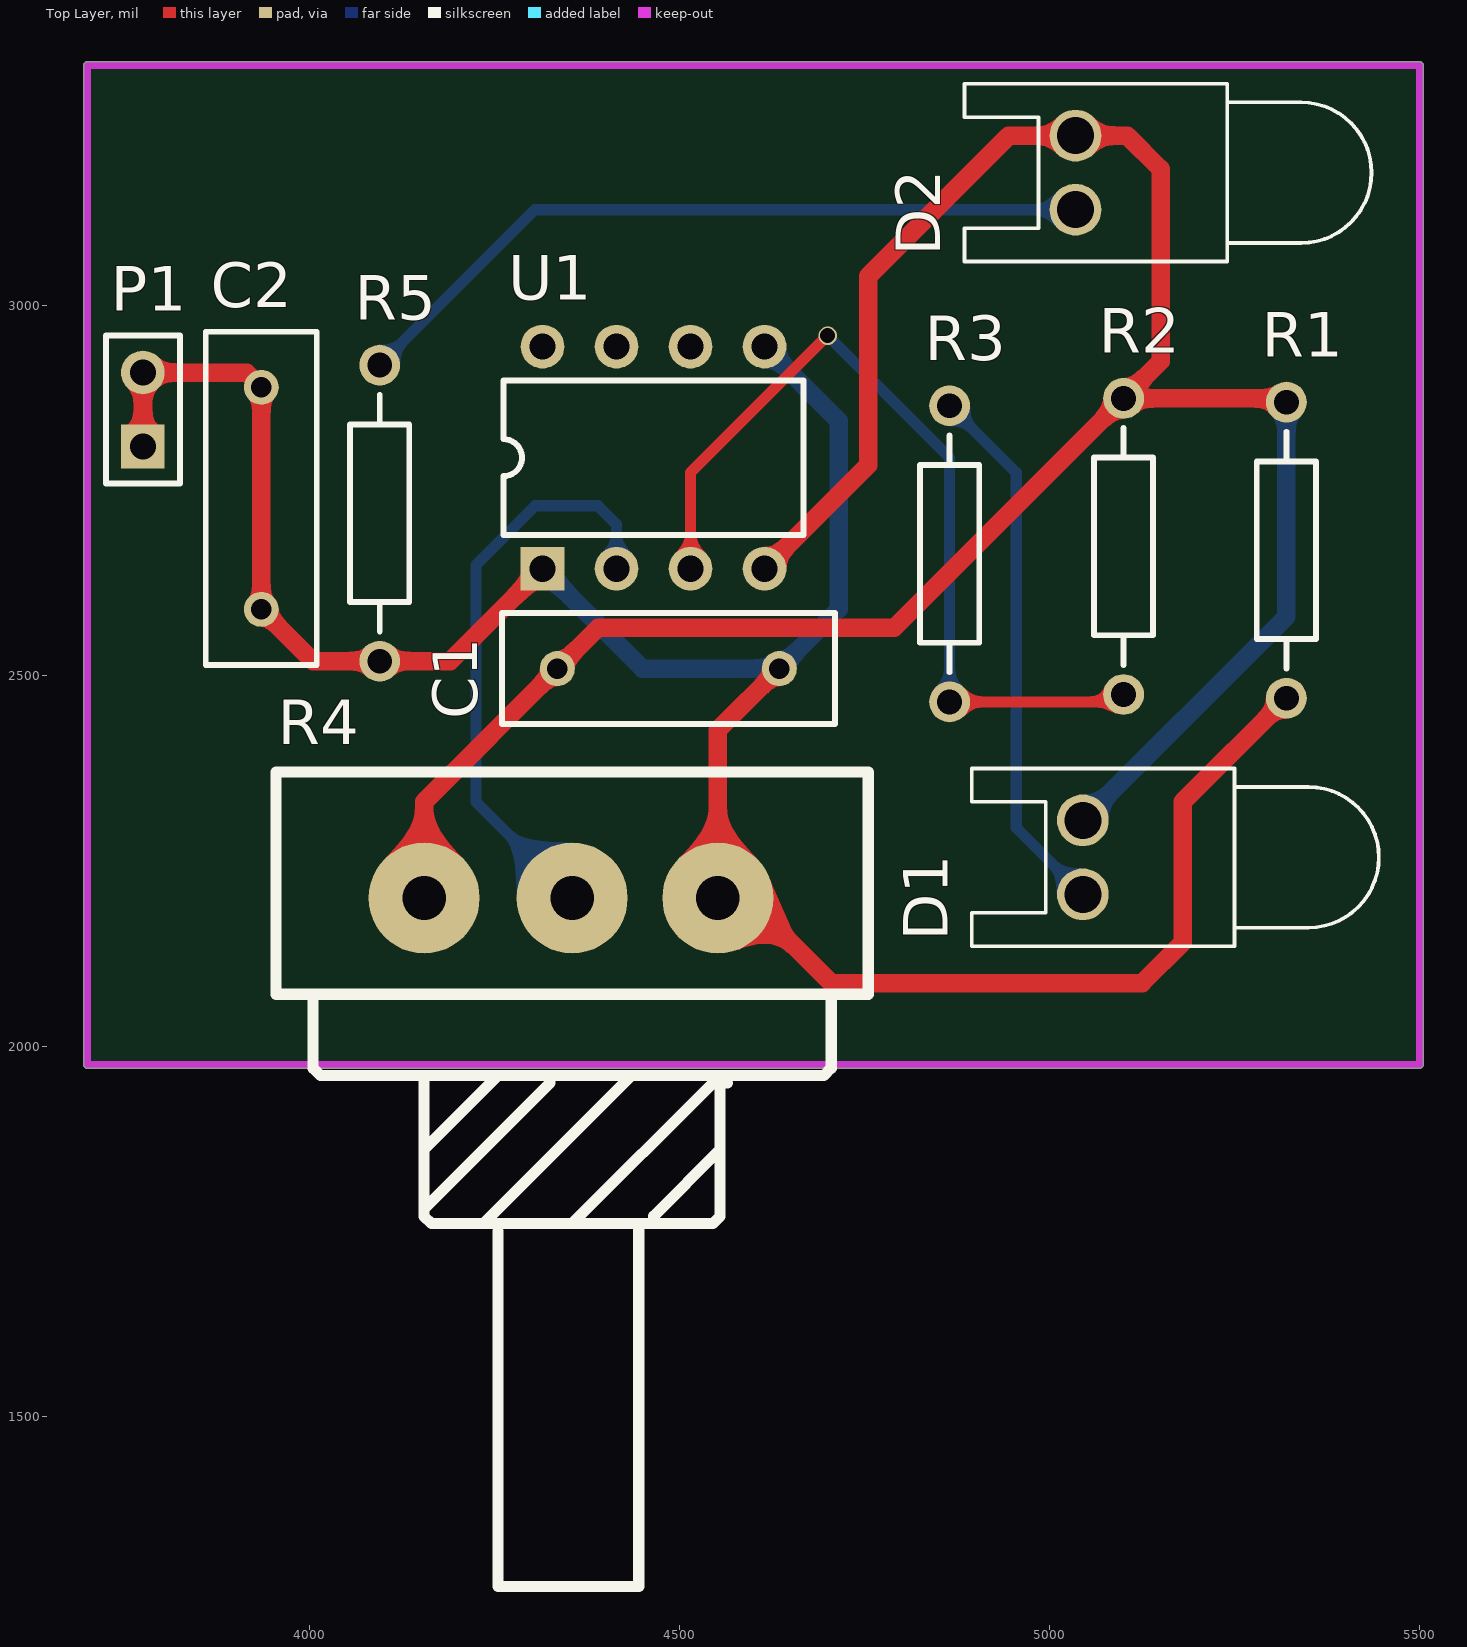
[diagram p0: Top Layer view]
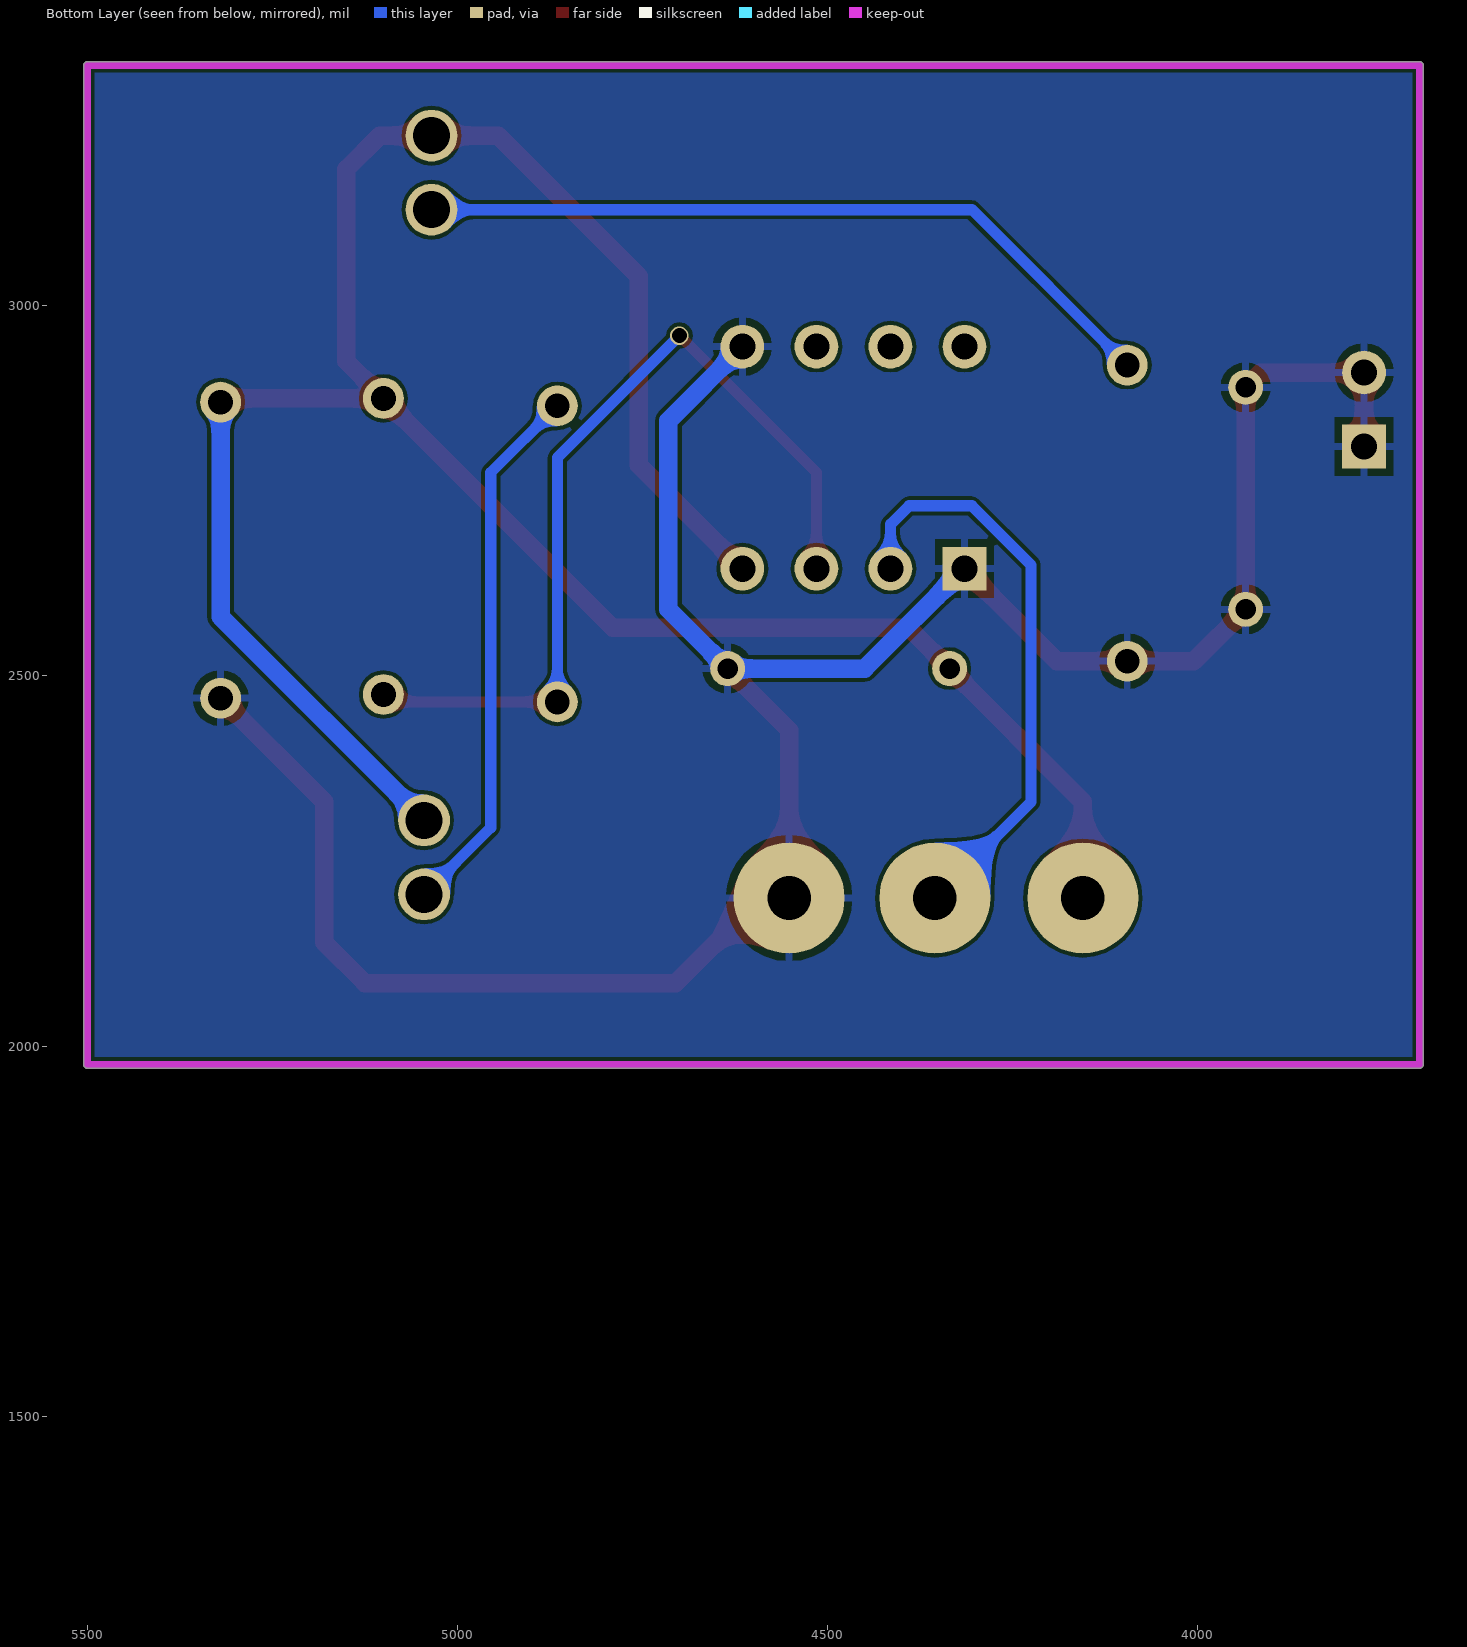
[diagram p1: Bottom Layer view, seen from below]
# Altium PCB MISC82777.PcbDoc
Units mil, origin at the board's own origin, x right, y up, seen from the top; angles counter-clockwise.
Board outline 1810.03 x 1360.03 mil, 2 copper layers (Top Layer, Bottom Layer); 11 components, 6 nets, 29 pads, 1 vias.

## Layer stack, top to bottom (the 12.6 mil dielectric is the usual default, probably not edited)
Top Solder: solder mask 0.4, Solder Resist, Dk 3.5
Top Layer: signal copper 1.4
Dielectric 1: dielectric 12.6, FR-4, Dk 4.8
Bottom Layer: signal copper 1.4
Bottom Solder: solder mask 0.4, Solder Resist, Dk 3.5

## Board outline
3694.99,1975 ccw(c3700,1975) 3700,1969.98 5500,1969.98 ccw(c5500,1975) 5505.02,1975 5505.02,3325 ccw(c5500,3325) 5500,3330.01 3700,3330.01 ccw(c3700,3325) 3694.99,3325

## Design rules (kind name [scope] priority, off if disabled: settings)
Clearance [All] p1: gap=5 ignorepadtopadclearanceinfootprint=FALSE except(0: Arc-Hole Track-Hole SMDPad-Hole THPad-Hole Via-Hole Fill-Hole Poly-Hole Region-Hole Text-Hole)
PolygonConnect [All] p1: connectstyle=Relief reliefconductorwidth=10 reliefentries=4 polygonreliefangle="90 Angle" airgapwidth=10
RoutingVias [All] p1: holewidth=28 width=50 viastyle="Through Hole" minholewidth=28 minwidth=50 maxholewidth=28 maxwidth=50
SolderMaskExpansion [All] p1: expansion=4
Width [All] p1: maxlimit=10000 minlimit=10 preferedwidth=10 minimp=50.000000 maximp=50.000000 favimp=50.000000
30 further rules are at their usual default settings.

## Components (designator, comment, footprint, x,y, rotation, side; value= is the part's Value field where it differs from the comment)
C1 "Cap" RAD-0.3 4485,2510 r180 top
C2 "Cap" RAD-0.3 3935,2740 r90 top
D1 "LED0" LED-0 5045,2255 r90 top
D2 "LED0" LED-0 5035,3180 r90 top
P1 "Header 2" HDR1X2 3775,2810 r90 top
R1 "Res2" AXIAL-0.4 5320,2670 r90 top
R2 "Res2" AXIAL-0.4 5100,2675 r90 top
R3 "Res2" AXIAL-0.4 4865,2665 r90 top
R4 "Sliding rheostat" 滑动变阻器 4355,1820 r0 top
R5 "Res2" AXIAL-0.4 4095,2720 r90 top
U1 "LM393" 626-05 4465,2795 r0 top

## Footprints (in the part's own frame and the unit in brackets; to place one, negate y for a bottom-side part, rotate by r counter-clockwise, add the part's x,y. Pads: shape width x height; smd on the part's side, far side on the other; paste and mask are expansions set on the pad)
626-05 [mm] "DIP; 8 Leads; Row Spacing 7.62 mm; Pitch 2.54 mm"
  rect 1.5x1.5 hole 0.9: 1(-3.81,-3.81)
  round 1.5 hole 0.9: 2(-1.27,-3.81) 3(1.27,-3.81) 4(3.81,-3.81) 5(3.81,3.81) 6(1.27,3.81) 7(-1.27,3.81) 8(-3.81,3.81)
  silkscreen extent -5.15,-2.65 5.15,2.65
AXIAL-0.4 [mm] "Axial Device, Thru-Hole; 2 Leads; 0.4 in Pin Spacing"
  round 1.4 hole 0.85: 1(-5.08,0) 2(5.08,0)
  silkscreen extent -4.06,-1.02 4.06,1.02
HDR1X2 [mm] "Connector; Header; 2 Position"
  rect 1.5x1.5 hole 0.9: 1(0,0)
  round 1.5 hole 0.9: 2(2.54,0)
  silkscreen extent -1.27,-1.27 3.81,1.27
LED-0 [mil] "LED; 2 Leads"
  round 70 hole 50: 1(50,0) 2(-50,0)
  silkscreen extent -120,-400 120,150
RAD-0.3 [mm] "Radial Cap, Thru-Hole; 2 Leads; 0.3 in Pin Spacing"
  round 1.2 hole 0.7: 1(-3.81,0) 2(3.81,0)
  silkscreen extent -5.71,-1.91 5.71,1.91
滑动变阻器 [mil]
  round 150 hole 59.06 paste+0 mask+4: 1(-200,380) 3(196.85,380)
  round 150 hole 59.05 paste+4 mask+4: 2(0,380)
  silkscreen extent -400,-550 400,550

## Part data
C1 C2: "Capacitor"
D1 D2: "Typical INFRARED GaAs LED"
P1: "Header, 2-Pin"
R1 R2 R3 R5: "Resistor"
R4: library part 滑动变阻器
U1: library part LM393N, "Dual Comparator"

## Via types
v1: diameter 25, hole 20, Top Layer to Bottom Layer, 1 vias

## Nets (pads, with @x,y where several pads share a name; then routed paths per layer and width w, separated by ;. In a path a pad name is that pad's centre, name@x,y a point inside that pad or via, vN(x,y) a via of type N, cw(c..) or ccw(c..) an arc to the next point about the centre after c; other vN are vias at no path point)
GND: C1.1 C2.1 C2.2 P1.1 P1.2 R1.1 R4.3 R5.1 U1.1 U1.5 | length 3345.5
  Top Layer w25: P1.1 P1.2 3915,2910 C2.2 C2.1 4005,2520 R5.1 4190,2520 U1.1 ; C1.1 4551.85,2426.85 R4.3 4590,2200 4705,2085 5125,2085 5180,2140 5180,2330 R1.1
  Bottom Layer w25: U1.1 4450,2510 C1.1 4715,2590 4715,2845 U1.5
NetD1_2: D1.2 R3.2 | length 734.6
  Bottom Layer w15: R3.2 4955,2775 4955,2295 D1.2
NetD2_2: D2.2 R5.2 | length 1027
  Bottom Layer w15: R5.2 4305,3130 D2.2
NetR2_1: R2.1 R3.1 U1.3 | length 1194.1
  Top Layer w15: U1.3 4515,2775 v1(4700,2960) ; R3.1 5090,2465 R2.1
  Bottom Layer w15: v1(4700,2960) 4865,2795 R3.1
NetR4_2: R4.2 U1.2 | length 797.3
  Bottom Layer w15: R4.2 4225,2330 4225,2650 4305,2730 4390,2730 4415,2705 U1.2
VCC: C1.2 D1.1 D2.1 R1.2 R2.2 R4.1 U1.4 | length 3477.8
  Top Layer w25: R4.1 4155,2330 C1.2 4390,2565 4790,2565 R2.2 ; U1.4 4755,2785 4755,3040 4945,3230 D2.1 5105,3230 5150,3185 5150,2925 R2.2 ; R1.2 5315,2875 R2.2
  Bottom Layer w25: D1.1 5320,2580 R1.2
pads on no net: U1.6 U1.7 U1.8

## Polygon pours and split planes (outlines as drawn)
GND on Bottom Layer "Top Layer-No Net" (solid, remove dead copper, pour order 2): 3570,3395 3580,3405 5695,3405 5695,1765 5680,1750 5670,1760 3605,1760

## Keep-outs
Keep-Out Layer:
  lines w10: 3700,1975 3700,3325 5475,3325 5500,3325 5500,1975 5480,1975 5465,1975 3700,1975